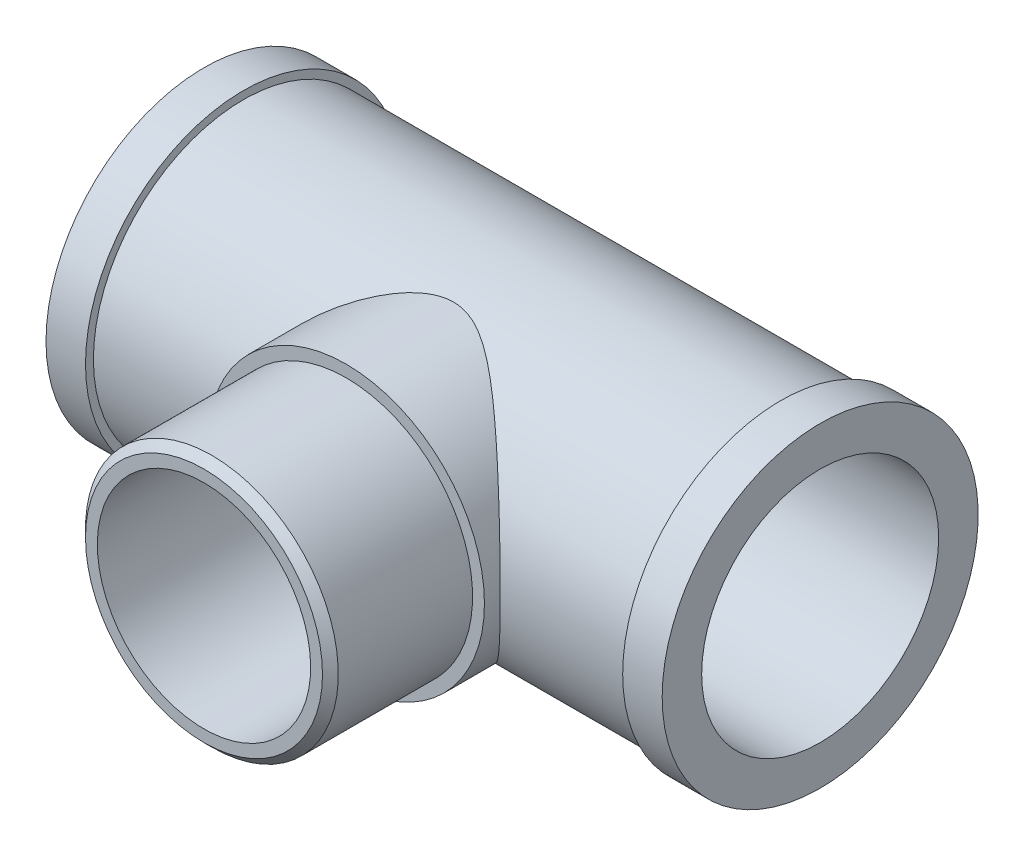
from build123d import *

# Parameters (mm, degrees)
SKETCH4_R          = 15
CUT_EXTRUDE1_DEPTH = 90.470665715
CUT_EXTRUDE2_REACH = 101.825
SKETCH5_R          = 13.5
CHAMFER1_SIZE      = 1


with BuildPart() as part:
    # Sketch1 → Revolve1 (revolve)
    with BuildSketch(Plane.XY, mode=Mode.PRIVATE) as revolve1_sk:
        Polygon((5, 19), (5, 20), (0, 20), (0, 15), (78, 15), (78, 20), (73, 20), (73, 19), align=None)
    revolve(revolve1_sk.sketch.rotate(Axis((0, 0, 0), (1, 0, 0)), 90), axis=Axis((0, 0, 0), (1, 0, 0)))

    # Sketch3 → Revolve2 (revolve)
    with BuildSketch(Plane(origin=(39, 0, 0), x_dir=(0, 0, -1), z_dir=(1, 0, 0)), mode=Mode.PRIVATE) as revolve2_sk:
        Polygon((-39, -13.5), (-39, -16), (-21, -16), (-21, -17.5), (-6.538348415, -17.5), (-6.538348415, -13.5), align=None)
    revolve(revolve2_sk.sketch.rotate(Axis((39, 0, 0), (0, 0, 1)), 180), axis=Axis((39, 0, 0), (0, 0, 1)))

    # Sketch4 → Cut-Extrude1 (cut, through all)
    with BuildSketch(Plane.ZY):
        Circle(SKETCH4_R)
    extrude(amount=-CUT_EXTRUDE1_DEPTH, mode=Mode.SUBTRACT)

    # Sketch5 → Cut-Extrude2 (cut, up to next)
    with BuildSketch(Plane.XY.offset(39), mode=Mode.PRIVATE) as cut_extrude2_sk1:
        with Locations(Location((39, 0, 0), (0, 0, 90))):
            Circle(SKETCH5_R)
    cut_extrude2_tool1 = extrude(cut_extrude2_sk1.sketch, amount=-CUT_EXTRUDE2_REACH, mode=Mode.PRIVATE) & part.part
    add(cut_extrude2_tool1.solids().sort_by_distance((39, 0, 39))[0], mode=Mode.SUBTRACT)

    # Chamfer1
    chamfer1_edges = [part.edges().sort_by_distance(p)[0] for p in [
        (39, -16, 39),
    ]]
    chamfer(chamfer1_edges, length=CHAMFER1_SIZE)


solid = part.part
